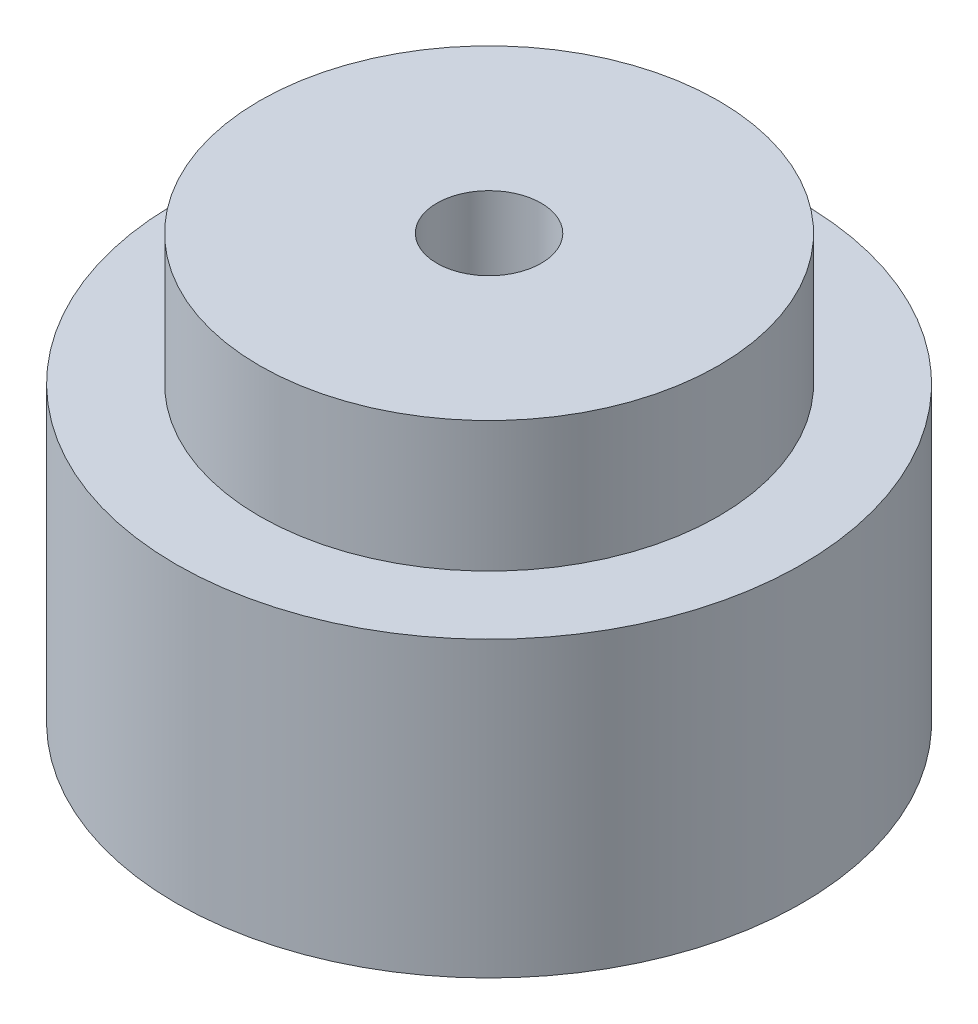
SolidWorks part; units mm, degrees
material "普通碳钢"
ref_plane "前视" through (0, 0, 0) normal (0, 0, 1) x (1, 0, 0)
ref_plane "上视" through (0, 0, 0) normal (0, 1, 0) x (1, 0, 0)
ref_plane "右视" through (0, 0, 0) normal (1, 0, 0) x (0, 0, -1)
sketch "草图1" plane through (0, 0, 0) normal (0, 0, 1) x (1, 0, 0)
  line L0 (-81.8, 0) -> (87.2, 0) construction
  line L1 (0, 61.8) -> (0, -63.2) construction
  line L2 (-4, 32.5) -> (-17.6, 32.5)
  line L3 (-17.6, 32.5) -> (-17.6, 22.5)
  line L4 (-17.6, 22.5) -> (-24, 22.5)
  line L5 (-24, 22.5) -> (-24, 0)
  line L6 (-24, 0) -> (-20, 0)
  line L8 (-4, 20.6) -> (-4, 32.5)
  line L9 (-4, 20.6) -> (-20, 15)
  line L10 (-20, 15) -> (-20, 0)
  dimension "D1" = 10
  dimension "D2" = 4
  dimension "D3" = 11.9
  dimension "D4" = 20
  dimension "D5" = 17.5
  dimension "D6" = 32.5
  dimension "D7" = 24
revolve "旋转1" add sketch "草图1" angle 360 about L1
